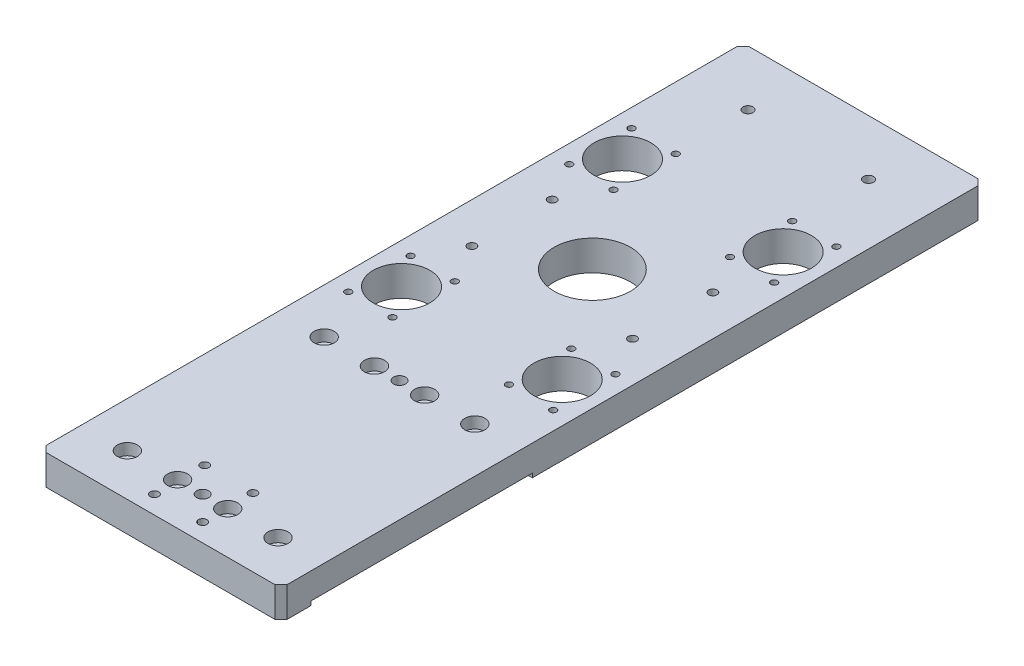
SolidWorks part; units mm, degrees
material "A6061 T6"
ref_plane "前视基准面" through (0, 0, 0) normal (0, 0, 1) x (1, 0, 0)
ref_plane "上视基准面" through (0, 0, 0) normal (0, 1, 0) x (1, 0, 0)
ref_plane "右视基准面" through (0, 0, 0) normal (1, 0, 0) x (0, 0, -1)
sketch "草图1" plane through (0, 0, 0) normal (0, 1, 0) x (1, 0, 0)
  line L1 (-60, 175) -> (60, 175)
  line L2 (-60, 175) -> (-60, -175)
  line L3 (-60, -175) -> (60, -175)
  line L4 (60, 175) -> (60, -175)
  line L5 (-60, 175) -> (60, -175) construction
  line L6 (-60, -175) -> (60, 175) construction
  point P0 (0, 0)
  dimension "D1" = 120
  dimension "D2" = 350
extrude "凸台-拉伸1" add sketch "草图1" along normal blind 15
sketch "草图3" plane through (0, 0, 0) normal (0, -1, 0) x (1, 0, 0)
  line L0 (-60, -175) -> (-60, 175) construction
  line L1 (-60, 160.1) -> (60, 160.1)
  line L2 (-60, 160.1) -> (-60, 49.9)
  line L3 (-60, 49.9) -> (60, 49.9)
  line L4 (60, 160.1) -> (60, 49.9)
  line L5 (60, 175) -> (60, -175) construction
  line L6 (-60, 175) -> (60, 175) construction
  dimension "D1" = 14.9
  dimension "D2" = 110.2
extrude "切除-拉伸1" cut sketch "草图3" against normal blind 2
hole_wizard "打孔尺寸(%根据)内六角圆柱头螺钉的类型0" positions "草图4" profile "草图5" counterbore size "M5" standard "GB"
sketch "草图4" plane through (0, 15, 0) normal (0, 1, 0) x (1, 0, 0)
  point P0 (-37.5, -154)
  point P3 (-12.5, -154)
  point P6 (12.5, -154)
  point P9 (37.5, -154)
  point P12 (-37.5, -56)
  point P15 (-12.5, -56)
  point P18 (12.5, -56)
  point P21 (37.5, -56)
sketch "草图5" plane through (-37.5, 15, 154) normal (1, 0, 0) x (0, 0, 1)
  line L0 (0, 0) -> (0, 26.6524)
  line L1 (0, 26.6524) -> (2.75, 25)
  line L2 (2.75, 25) -> (2.75, 5.7)
  line L3 (2.75, 5.7) -> (5, 5.7)
  line L4 (5, 5.7) -> (5, 0)
  line L5 (5, 0) -> (0, 0)
  line L10 (0, 26.6524) -> (-2.75, 25) construction
  line L11 (0, -6.35) -> (0, 107.95) construction
  dimension "孔直径" = 5.5
  dimension "孔深度" = 25
  dimension "柱形沉头孔直径" = 10
  dimension "柱形沉头孔深度" = 5.7
  dimension "导头角度" = 118
hole_wizard "大小mm 暗销孔1" positions "草图6" profile "草图7" hole size "Ø6.0" standard "GB"
sketch "草图6" plane through (0, 15, 0) normal (0, 1, 0) x (1, 0, 0)
  point P0 (0, -154)
  point P3 (0, -56)
sketch "草图7" plane through (0, 15, 154) normal (1, 0, 0) x (0, 0, 1)
  line L0 (0, 0) -> (0, 26.8026)
  line L1 (0, 26.8026) -> (3, 25)
  line L2 (3, 25) -> (3, 0)
  line L5 (3, 0) -> (0, 0)
  line L10 (0, 26.8026) -> (-3, 25) construction
  line L11 (0, -6.35) -> (0, 107.95) construction
  dimension "孔直径" = 6
  dimension "孔深度" = 25
  dimension "导头角度" = 118
chamfer "倒角1" distance 3 angle 45 4 edges at (-60, 7.5, -175) (60, 7.5, -175) (60, 7.5, 175) (-60, 7.5, 175)
sketch "草图8" plane through (0, 15, 0) normal (0, 1, 0) x (1, 0, 0)
  line L0 (57, 175) -> (-57, 175) construction
  circle A0 centre (0, 40) radius 19
  dimension "D1" = 38
  dimension "D2" = 135
extrude "切除-拉伸2" cut sketch "草图8" against normal blind 20
sketch "草图9" plane through (0, 15, 0) normal (0, 1, 0) x (1, 0, 0)
  line L0 (57, 175) -> (-57, 175) construction
  line L1 (60, -172) -> (60, 172) construction
  line L2 (-60, 172) -> (-60, -172) construction
  circle A0 centre (40, -15) radius 14.1
  circle A1 centre (40, 95) radius 14.1
  circle A3 centre (-40, -15) radius 14.1
  circle A4 centre (-40, 95) radius 14.1
  dimension "D1" = 28.2
  dimension "D2" = 110
  dimension "D3" = 80
  dimension "D4" = 20
  dimension "D5" = 20
extrude "切除-拉伸3" cut sketch "草图9" against normal blind 20
hole_wizard "大小mm 暗销孔2" positions "草图14" profile "草图15" hole size "Ø5.0" standard "GB"
sketch "草图14" plane through (0, 15, 0) normal (0, 1, 0) x (1, 0, 0)
  point P0 (30, 147.5)
  point P3 (-30, 147.5)
sketch "草图15" plane through (30, 15, -147.5) normal (1, 0, 0) x (0, 0, 1)
  line L0 (0, 0) -> (0, 21.5022)
  line L1 (0, 21.5022) -> (2.5, 20)
  line L2 (2.5, 20) -> (2.5, 0)
  line L5 (2.5, 0) -> (0, 0)
  line L10 (0, 21.5022) -> (-2.5, 20) construction
  line L11 (0, -6.35) -> (0, 107.95) construction
  dimension "孔直径" = 5
  dimension "孔深度" = 20
  dimension "导头角度" = 118
hole_wizard "M5 螺纹孔1" positions "草图16" profile "草图17" tap size "M5" standard "GB"
sketch "草图16" plane through (0, 0, 0) normal (0, -1, 0) x (-1, 0, 0)
  point P0 (40, 20)
  point P3 (-40, 20)
  point P6 (40, 60)
  point P9 (-40, 60)
sketch "草图17" plane through (-40, 0, -20) normal (1, 0, 0) x (0, 0, -1)
  line L0 (0, 0) -> (0, 21.2618)
  line L1 (0, 21.2618) -> (2.1, 20)
  line L2 (2.1, 20) -> (2.1, 0)
  line L5 (2.1, 0) -> (0, 0)
  line L10 (0, 21.2618) -> (-2.1, 20) construction
  line L11 (0, -6.35) -> (0, 107.95) construction
  dimension "螺纹孔钻头直径" = 4.2
  dimension "螺纹孔钻头深度" = 20
  dimension "导头角度" = 118
cosmetic thread "孔螺蚊线5" parameters "D1"=10, "D2"=5
cosmetic thread "孔螺蚊线6" parameters "D1"=10, "D2"=5
cosmetic thread "孔螺蚊线7" parameters "D1"=10, "D2"=5
cosmetic thread "孔螺蚊线8" parameters "D1"=10, "D2"=5
hole_wizard "M4 螺纹孔1" positions "草图18" profile "草图19" tap size "M4" standard "GB"
sketch "草图18" plane through (0, 15, 0) normal (0, 1, 0) x (1, 0, 0)
  point P0 (51, -30.5)
  point P3 (29, -30.5)
  point P6 (51, 0.5)
  point P9 (29, 0.5)
  point P12 (-51, -30.5)
  point P15 (-29, -30.5)
  point P18 (-29, 0.5)
  point P21 (-51, 0.5)
  point P24 (51, 79.5)
  point P27 (29, 79.5)
  point P30 (51, 110.5)
  point P33 (29, 110.5)
  point P36 (-29, 79.5)
  point P39 (-51, 79.5)
  point P42 (-29, 110.5)
  point P45 (-51, 110.5)
sketch "草图19" plane through (51, 15, 30.5) normal (1, 0, 0) x (0, 0, 1)
  line L0 (0, 0) -> (0, 32.9914)
  line L1 (0, 32.9914) -> (1.65, 32)
  line L2 (1.65, 32) -> (1.65, 0)
  line L5 (1.65, 0) -> (0, 0)
  line L10 (0, 32.9914) -> (-1.65, 32) construction
  line L11 (0, -6.35) -> (0, 107.95) construction
  dimension "螺纹孔钻头直径" = 3.3
  dimension "螺纹孔钻头深度" = 32
  dimension "导头角度" = 118
cosmetic thread "孔螺蚊线9" parameters "D1"=8, "D2"=4
cosmetic thread "孔螺蚊线10" parameters "D1"=8, "D2"=4
cosmetic thread "孔螺蚊线11" parameters "D1"=8, "D2"=4
cosmetic thread "孔螺蚊线12" parameters "D1"=8, "D2"=4
cosmetic thread "孔螺蚊线13" parameters "D1"=8, "D2"=4
cosmetic thread "孔螺蚊线14" parameters "D1"=8, "D2"=4
cosmetic thread "孔螺蚊线15" parameters "D1"=8, "D2"=4
cosmetic thread "孔螺蚊线16" parameters "D1"=8, "D2"=4
cosmetic thread "孔螺蚊线17" parameters "D1"=8, "D2"=4
cosmetic thread "孔螺蚊线18" parameters "D1"=8, "D2"=4
cosmetic thread "孔螺蚊线19" parameters "D1"=8, "D2"=4
cosmetic thread "孔螺蚊线20" parameters "D1"=8, "D2"=4
cosmetic thread "孔螺蚊线21" parameters "D1"=8, "D2"=4
cosmetic thread "孔螺蚊线22" parameters "D1"=8, "D2"=4
cosmetic thread "孔螺蚊线23" parameters "D1"=8, "D2"=4
cosmetic thread "孔螺蚊线24" parameters "D1"=8, "D2"=4
hole_wizard "M5 螺纹孔2" positions "草图20" profile "草图21" tap size "M5" standard "GB"
sketch "草图20" plane through (0, 15, 0) normal (0, 1, 0) x (1, 0, 0)
  point P0 (-12, -141)
  point P3 (12, -141)
  point P6 (-12, -166)
  point P9 (12, -166)
sketch "草图21" plane through (-12, 15, 141) normal (1, 0, 0) x (0, 0, 1)
  line L0 (0, 0) -> (0, 21.2618)
  line L1 (0, 21.2618) -> (2.1, 20)
  line L2 (2.1, 20) -> (2.1, 0)
  line L5 (2.1, 0) -> (0, 0)
  line L10 (0, 21.2618) -> (-2.1, 20) construction
  line L11 (0, -6.35) -> (0, 107.95) construction
  dimension "螺纹孔钻头直径" = 4.2
  dimension "螺纹孔钻头深度" = 20
  dimension "导头角度" = 118
cosmetic thread "孔螺蚊线25" parameters "D1"=10, "D2"=5
cosmetic thread "孔螺蚊线26" parameters "D1"=10, "D2"=5
cosmetic thread "孔螺蚊线27" parameters "D1"=10, "D2"=5
cosmetic thread "孔螺蚊线28" parameters "D1"=10, "D2"=5
